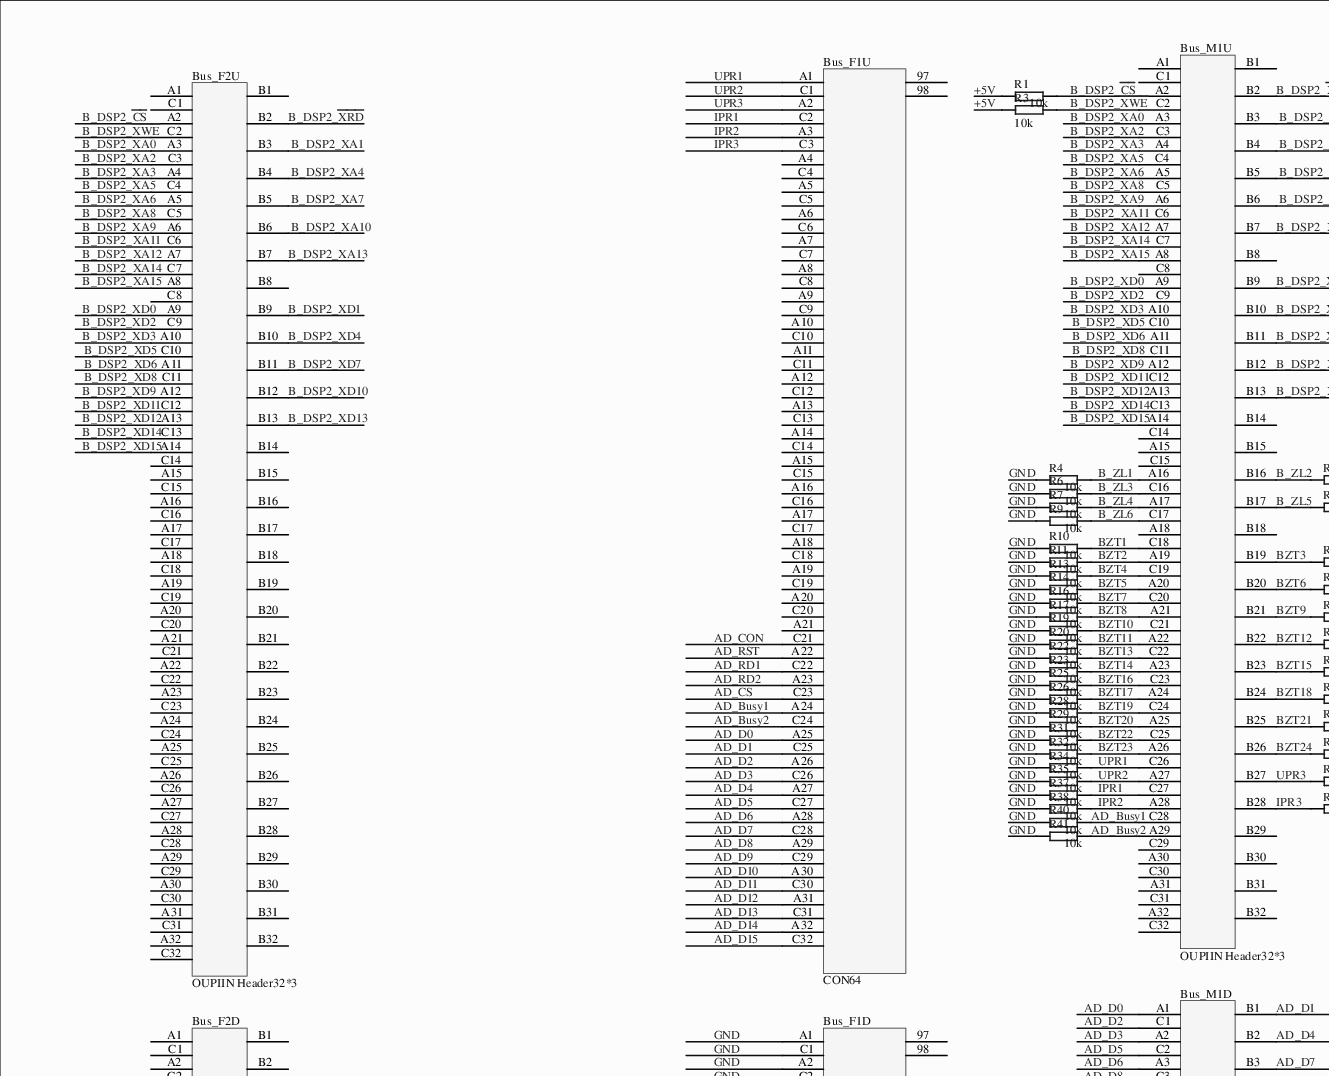
[diagram p0: MISC67337.SchDoc, top left]
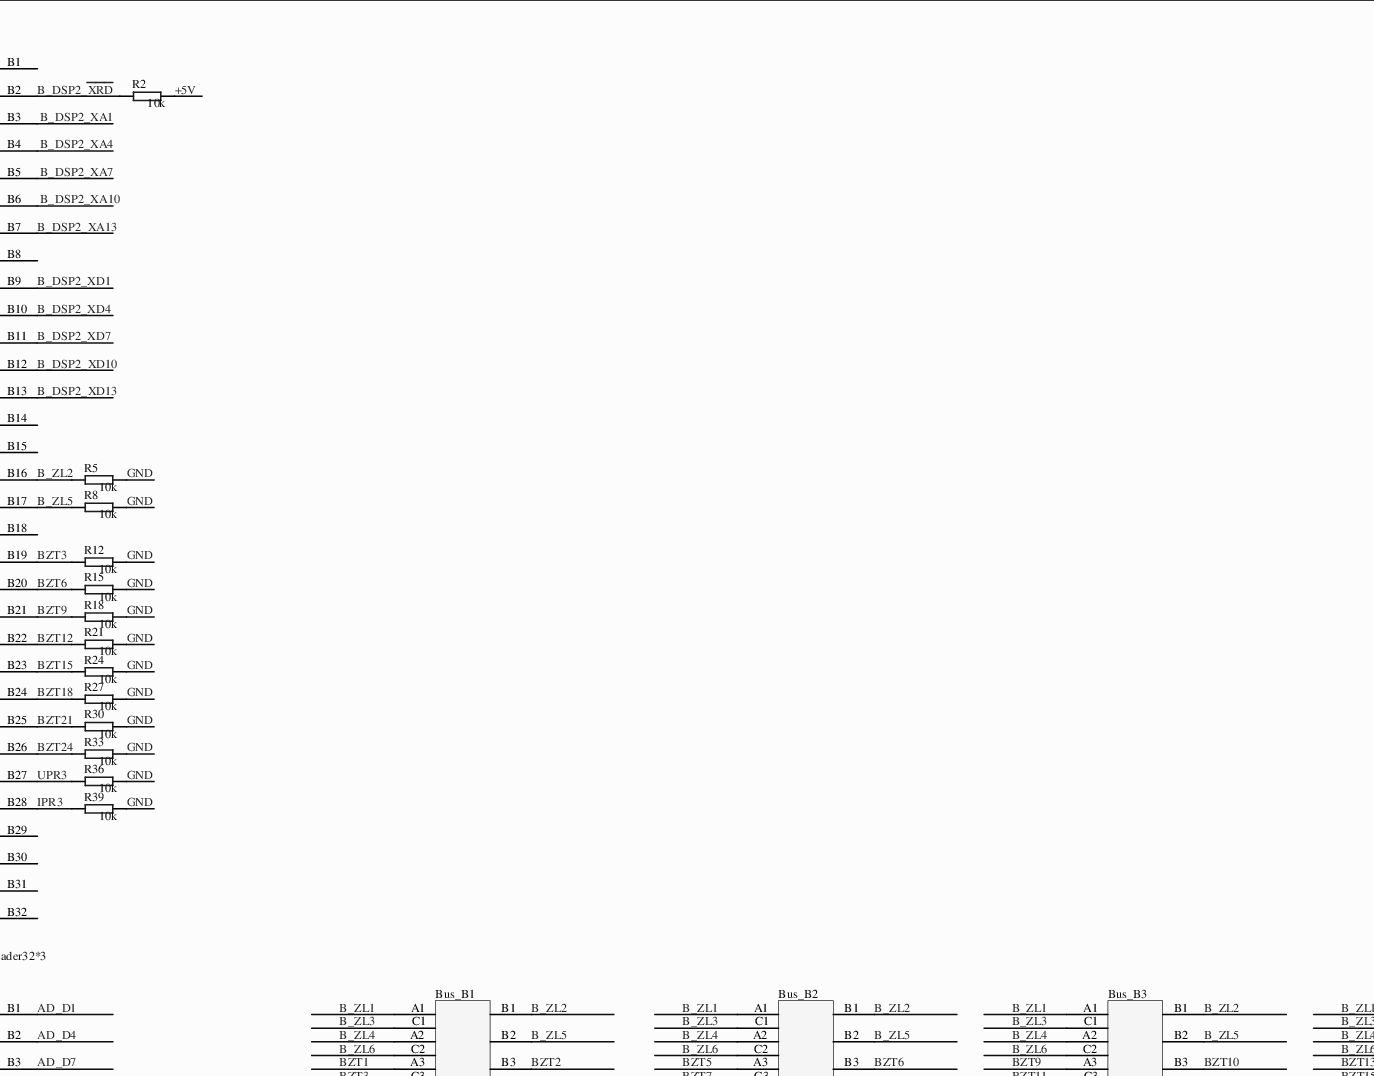
[diagram p1: MISC67337.SchDoc, top middle]
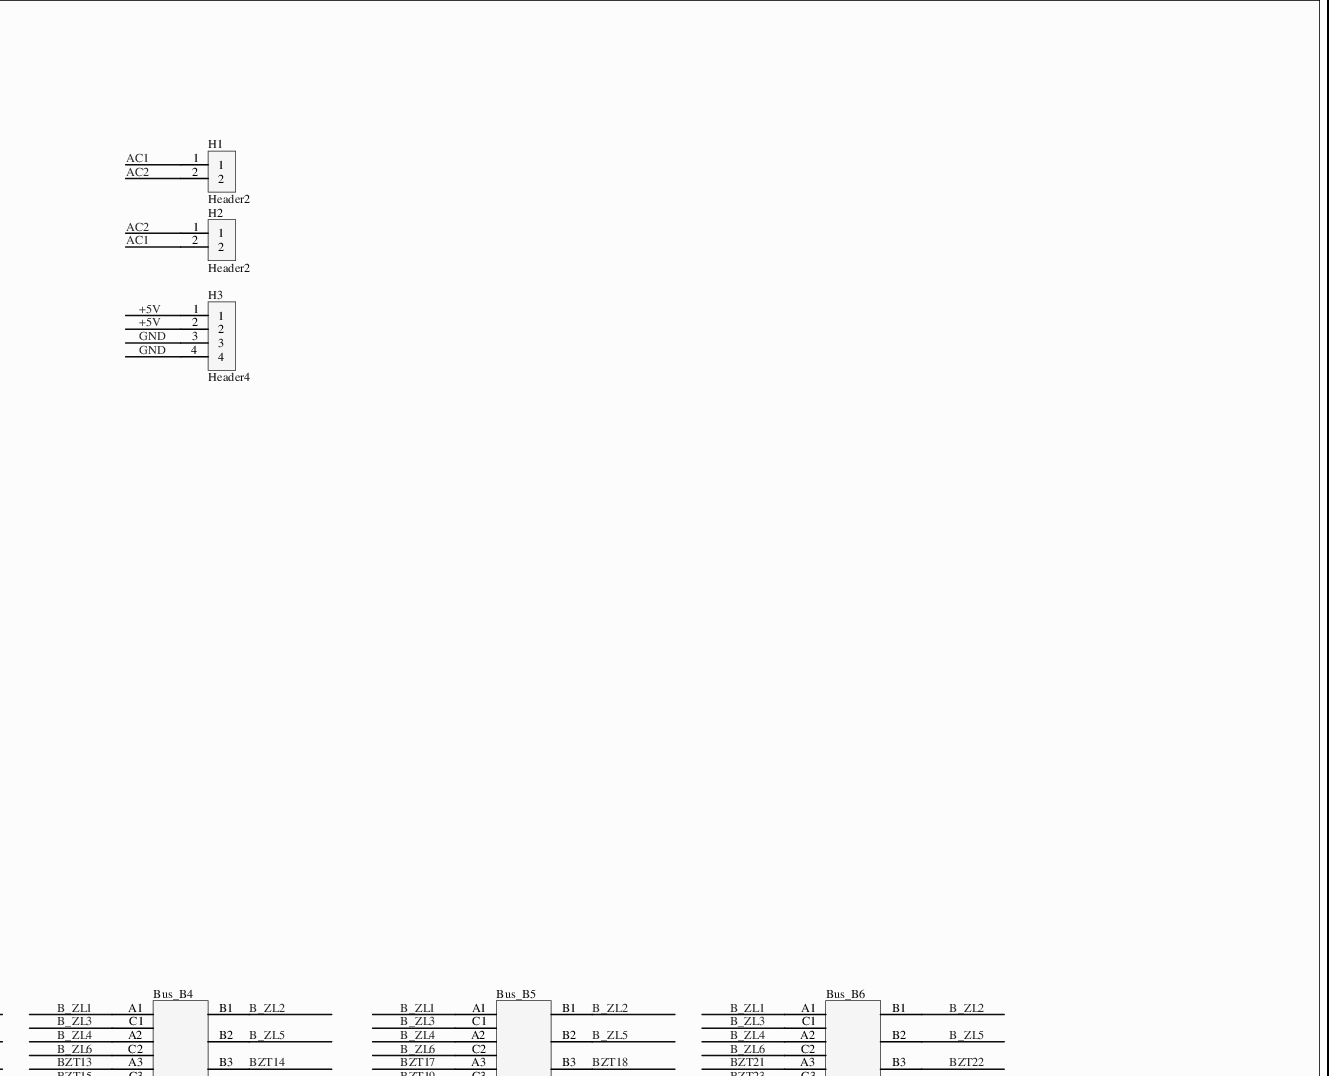
[diagram p2: MISC67337.SchDoc, top right]
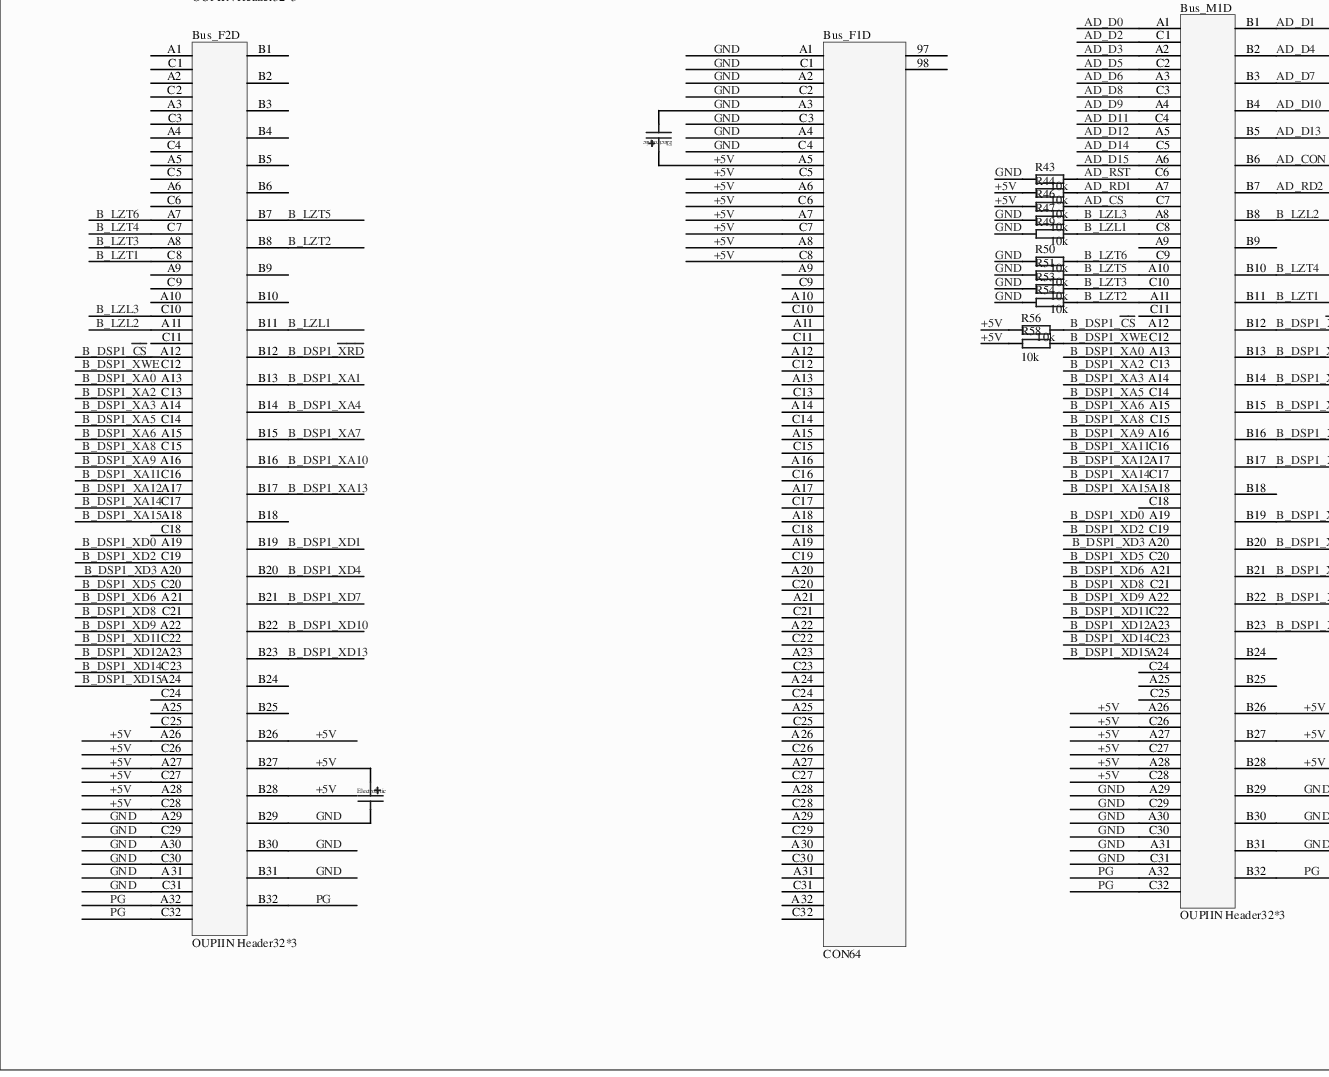
[diagram p3: MISC67337.SchDoc, bottom left]
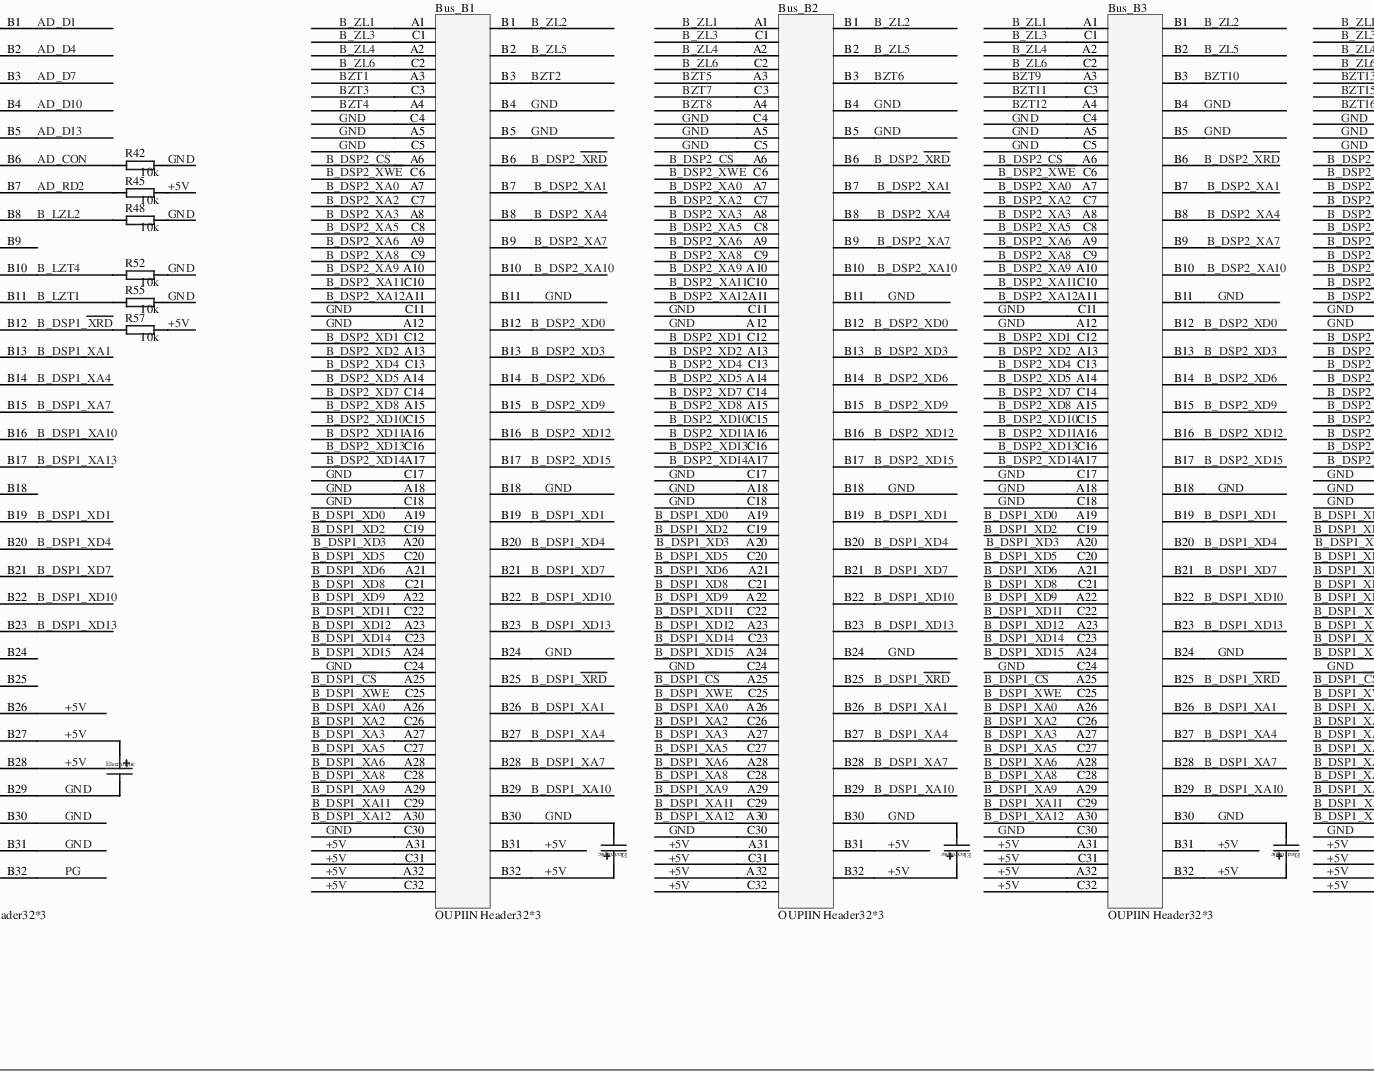
[diagram p4: MISC67337.SchDoc, bottom middle]
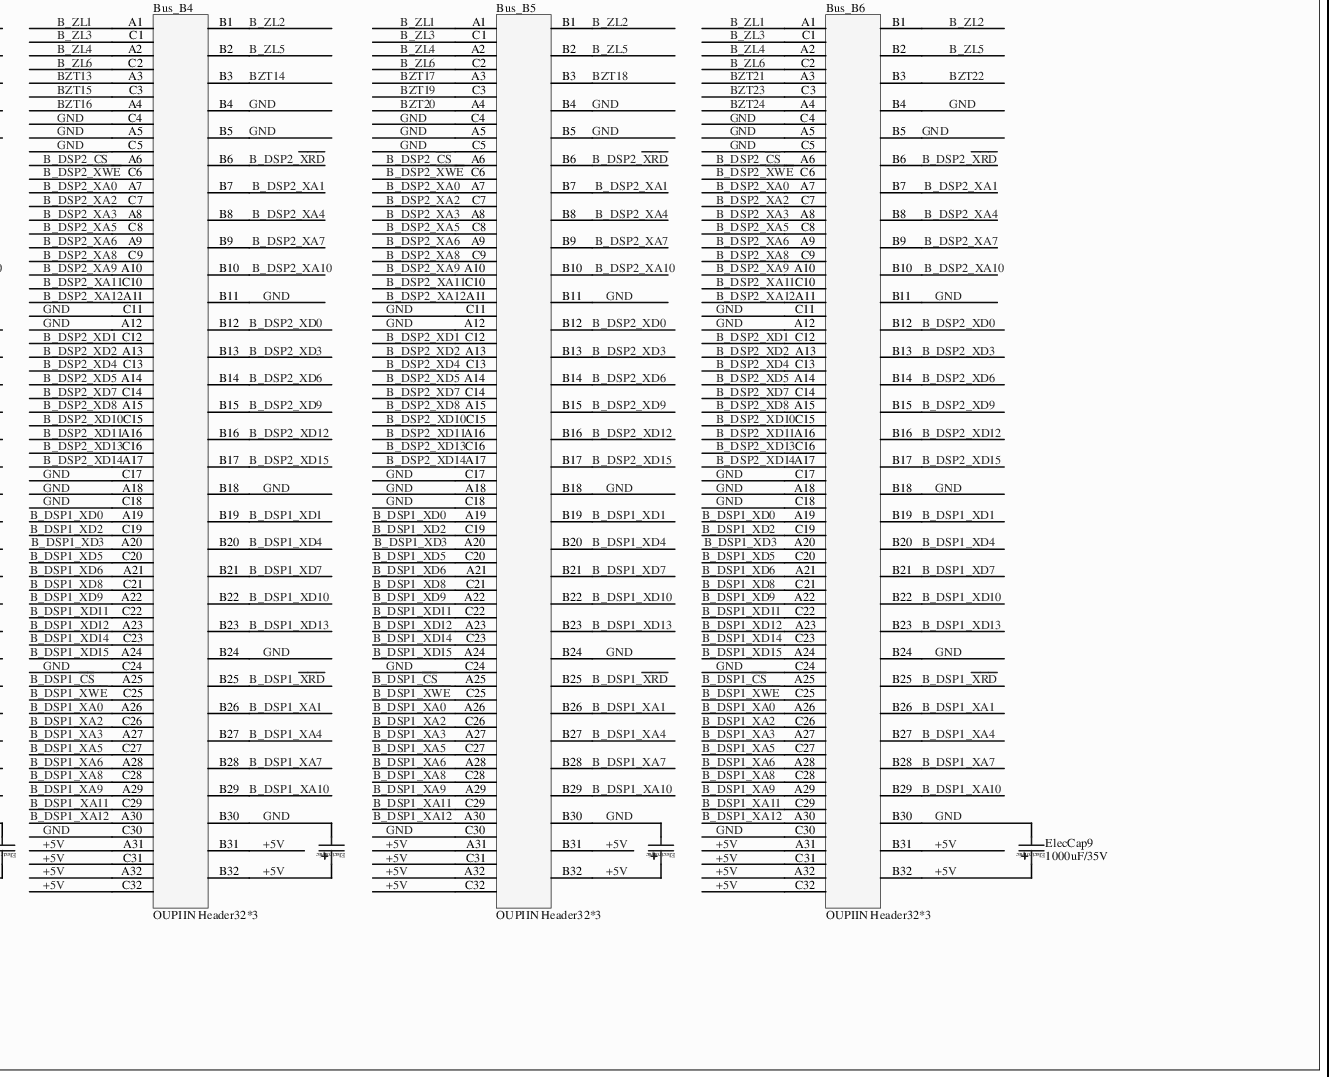
[diagram p5: MISC67337.SchDoc, bottom right]
# Altium project MISC67337.PrjPcb
1 sheet, 82 parts. Net scope: global (net labels, ports and power ports of the same name join across sheets).
Board file: MISC67337.PcbDoc

## Sheet MISC67337.SchDoc
size 711 x 381 mm; SheetNumber: 0; SheetTotal: 0

### Parts
Bus_B1  OUPIIN Header32*3  [OUPIINBus32*3_zhili]
Bus_B2  OUPIIN Header32*3  [OUPIINBus32*3_zhili]
Bus_B3  OUPIIN Header32*3  [OUPIINBus32*3_zhili]
Bus_B4  OUPIIN Header32*3  [OUPIINBus32*3_zhili]
Bus_B5  OUPIIN Header32*3  [OUPIINBus32*3_zhili]
Bus_B6  OUPIIN Header32*3  [OUPIINBus32*3_zhili]
Bus_F1D  CON64  [OUPIINBus32*2_zhili]
Bus_F1U  CON64  [OUPIINBus32*2_zhili]
Bus_F2D  OUPIIN Header32*3  [OUPIINBus32*3_zhili]
Bus_F2U  OUPIIN Header32*3  [OUPIINBus32*3_zhili]
Bus_M1D  OUPIIN Header32*3  [OUPIINBus32*3_zhili]
Bus_M1U  OUPIIN Header32*3  [OUPIINBus32*3_zhili]
ElecCap1  1000uF/35V  [1000UF/35V]  (value not drawn)
ElecCap2  1000uF/35V  [1000UF/35V]  (value not drawn)
ElecCap3  1000uF/35V  [1000UF/35V]  (value not drawn)
ElecCap4  1000uF/35V  [1000UF/35V]  (value not drawn)
ElecCap5  1000uF/35V  [1000UF/35V]  (value not drawn)
ElecCap6  1000uF/35V  [1000UF/35V]  (value not drawn)
ElecCap7  1000uF/35V  [1000UF/35V]  (value not drawn)
ElecCap8  1000uF/35V  [1000UF/35V]  (value not drawn)
ElecCap9  1000uF/35V  [1000UF/35V]
H1  Header2  [EDGCon_2p_5.08mm]
H2  Header2  [EDGCON_2p_5.08mm_ear]
H3  Header4  [EDGCON_4p_5.08mm]
R1  10k  [0603]
R2  10k  [0603]
R3  10k  [0603]
R4  10k  [0603]
R5  10k  [0603]
R6  10k  [0603]
R7  10k  [0603]
R8  10k  [0603]
R9  10k  [0603]
R10  10k  [0603]
R11  10k  [0603]
R12  10k  [0603]
R13  10k  [0603]
R14  10k  [0603]
R15  10k  [0603]
R16  10k  [0603]
R17  10k  [0603]
R18  10k  [0603]
R19  10k  [0603]
R20  10k  [0603]
R21  10k  [0603]
R22  10k  [0603]
R23  10k  [0603]
R24  10k  [0603]
R25  10k  [0603]
R26  10k  [0603]
R27  10k  [0603]
R28  10k  [0603]
R29  10k  [0603]
R30  10k  [0603]
R31  10k  [0603]
R32  10k  [0603]
R33  10k  [0603]
R34  10k  [0603]
R35  10k  [0603]
R36  10k  [0603]
R37  10k  [0603]
R38  10k  [0603]
R39  10k  [0603]
R40  10k  [0603]
R41  10k  [0603]
R42  10k  [0603]
R43  10k  [0603]
R44  10k  [0603]
R45  10k  [0603]
R46  10k  [0603]
R47  10k  [0603]
R48  10k  [0603]
R49  10k  [0603]
R50  10k  [0603]
R51  10k  [0603]
R52  10k  [0603]
R53  10k  [0603]
R54  10k  [0603]
R55  10k  [0603]
R56  10k  [0603]
R57  10k  [0603]
R58  10k  [0603]

### Nets
+5V: Bus_B1.A31 Bus_B1.A32 Bus_B1.B31 Bus_B1.B32 Bus_B1.C31 Bus_B1.C32 Bus_B2.A31 Bus_B2.A32 Bus_B2.B31 Bus_B2.B32 Bus_B2.C31 Bus_B2.C32 Bus_B3.A31 Bus_B3.A32 Bus_B3.B31 Bus_B3.B32 Bus_B3.C31 Bus_B3.C32 Bus_B4.A31 Bus_B4.A32 Bus_B4.B31 Bus_B4.B32 Bus_B4.C31 Bus_B4.C32 Bus_B5.A31 Bus_B5.A32 Bus_B5.B31 Bus_B5.B32 Bus_B5.C31 Bus_B5.C32 Bus_B6.A31 Bus_B6.A32 Bus_B6.B31 Bus_B6.B32 Bus_B6.C31 Bus_B6.C32 Bus_F1D.A5 Bus_F1D.A6 Bus_F1D.A7 Bus_F1D.A8 Bus_F1D.C5 Bus_F1D.C6 Bus_F1D.C7 Bus_F1D.C8 Bus_F2D.A26 Bus_F2D.A27 Bus_F2D.A28 Bus_F2D.B26 Bus_F2D.B27 Bus_F2D.B28 Bus_F2D.C26 Bus_F2D.C27 Bus_F2D.C28 Bus_M1D.A26 Bus_M1D.A27 Bus_M1D.A28 Bus_M1D.B26 Bus_M1D.B27 Bus_M1D.B28 Bus_M1D.C26 Bus_M1D.C27 Bus_M1D.C28 ElecCap1.1 ElecCap2.1 ElecCap3.1 ElecCap4.1 ElecCap5.1 ElecCap6.1 ElecCap7.1 ElecCap8.1 ElecCap9.1 H3.1 H3.2 R1.1 R2.2 R3.1 R44.1 R45.2 R46.1 R56.1 R57.2 R58.1
AC1: H1.1 H2.2
AC2: H1.2 H2.1
AD_Busy1: Bus_F1U.A24 Bus_M1U.C28 R40.2
AD_Busy2: Bus_F1U.C24 Bus_M1U.A29 R41.2
AD_CON: Bus_F1U.C21 Bus_M1D.B6 R42.1
AD_CS: Bus_F1U.C23 Bus_M1D.C7 R46.2
AD_D0: Bus_F1U.A25 Bus_M1D.A1
AD_D1: Bus_F1U.C25 Bus_M1D.B1
AD_D2: Bus_F1U.A26 Bus_M1D.C1
AD_D3: Bus_F1U.C26 Bus_M1D.A2
AD_D4: Bus_F1U.A27 Bus_M1D.B2
AD_D5: Bus_F1U.C27 Bus_M1D.C2
AD_D6: Bus_F1U.A28 Bus_M1D.A3
AD_D7: Bus_F1U.C28 Bus_M1D.B3
AD_D8: Bus_F1U.A29 Bus_M1D.C3
AD_D9: Bus_F1U.C29 Bus_M1D.A4
AD_D10: Bus_F1U.A30 Bus_M1D.B4
AD_D11: Bus_F1U.C30 Bus_M1D.C4
AD_D12: Bus_F1U.A31 Bus_M1D.A5
AD_D13: Bus_F1U.C31 Bus_M1D.B5
AD_D14: Bus_F1U.A32 Bus_M1D.C5
AD_D15: Bus_F1U.C32 Bus_M1D.A6
AD_RD1: Bus_F1U.C22 Bus_M1D.A7 R44.2
AD_RD2: Bus_F1U.A23 Bus_M1D.B7 R45.1
AD_RST: Bus_F1U.A22 Bus_M1D.C6 R43.2
B_DSP1_~{CS}: Bus_B1.A25 Bus_B2.A25 Bus_B3.A25 Bus_B4.A25 Bus_B5.A25 Bus_B6.A25 Bus_F2D.A12 Bus_M1D.A12 R56.2
B_DSP1_~{XRD}: Bus_B1.B25 Bus_B2.B25 Bus_B3.B25 Bus_B4.B25 Bus_B5.B25 Bus_B6.B25 Bus_F2D.B12 Bus_M1D.B12 R57.1
B_DSP1_~{XWE}: Bus_B1.C25 Bus_B2.C25 Bus_B3.C25 Bus_B4.C25 Bus_B5.C25 Bus_B6.C25 Bus_F2D.C12 Bus_M1D.C12 R58.2
B_DSP1_XA0: Bus_B1.A26 Bus_B2.A26 Bus_B3.A26 Bus_B4.A26 Bus_B5.A26 Bus_B6.A26 Bus_F2D.A13 Bus_M1D.A13
B_DSP1_XA1: Bus_B1.B26 Bus_B2.B26 Bus_B3.B26 Bus_B4.B26 Bus_B5.B26 Bus_B6.B26 Bus_F2D.B13 Bus_M1D.B13
B_DSP1_XA2: Bus_B1.C26 Bus_B2.C26 Bus_B3.C26 Bus_B4.C26 Bus_B5.C26 Bus_B6.C26 Bus_F2D.C13 Bus_M1D.C13
B_DSP1_XA3: Bus_B1.A27 Bus_B2.A27 Bus_B3.A27 Bus_B4.A27 Bus_B5.A27 Bus_B6.A27 Bus_F2D.A14 Bus_M1D.A14
B_DSP1_XA4: Bus_B1.B27 Bus_B2.B27 Bus_B3.B27 Bus_B4.B27 Bus_B5.B27 Bus_B6.B27 Bus_F2D.B14 Bus_M1D.B14
B_DSP1_XA5: Bus_B1.C27 Bus_B2.C27 Bus_B3.C27 Bus_B4.C27 Bus_B5.C27 Bus_B6.C27 Bus_F2D.C14 Bus_M1D.C14
B_DSP1_XA6: Bus_B1.A28 Bus_B2.A28 Bus_B3.A28 Bus_B4.A28 Bus_B5.A28 Bus_B6.A28 Bus_F2D.A15 Bus_M1D.A15
B_DSP1_XA7: Bus_B1.B28 Bus_B2.B28 Bus_B3.B28 Bus_B4.B28 Bus_B5.B28 Bus_B6.B28 Bus_F2D.B15 Bus_M1D.B15
B_DSP1_XA8: Bus_B1.C28 Bus_B2.C28 Bus_B3.C28 Bus_B4.C28 Bus_B5.C28 Bus_B6.C28 Bus_F2D.C15 Bus_M1D.C15
B_DSP1_XA9: Bus_B1.A29 Bus_B2.A29 Bus_B3.A29 Bus_B4.A29 Bus_B5.A29 Bus_B6.A29 Bus_F2D.A16 Bus_M1D.A16
B_DSP1_XA10: Bus_B1.B29 Bus_B2.B29 Bus_B3.B29 Bus_B4.B29 Bus_B5.B29 Bus_B6.B29 Bus_F2D.B16 Bus_M1D.B16
B_DSP1_XA11: Bus_B1.C29 Bus_B2.C29 Bus_B3.C29 Bus_B4.C29 Bus_B5.C29 Bus_B6.C29 Bus_F2D.C16 Bus_M1D.C16
B_DSP1_XA12: Bus_B1.A30 Bus_B2.A30 Bus_B3.A30 Bus_B4.A30 Bus_B5.A30 Bus_B6.A30 Bus_F2D.A17 Bus_M1D.A17
B_DSP1_XA13: Bus_F2D.B17 Bus_M1D.B17
B_DSP1_XA14: Bus_F2D.C17 Bus_M1D.C17
B_DSP1_XA15: Bus_F2D.A18 Bus_M1D.A18
B_DSP1_XD0: Bus_B1.A19 Bus_B2.A19 Bus_B3.A19 Bus_B4.A19 Bus_B5.A19 Bus_B6.A19 Bus_F2D.A19 Bus_M1D.A19
B_DSP1_XD1: Bus_B1.B19 Bus_B2.B19 Bus_B3.B19 Bus_B4.B19 Bus_B5.B19 Bus_B6.B19 Bus_F2D.B19 Bus_M1D.B19
B_DSP1_XD2: Bus_B1.C19 Bus_B2.C19 Bus_B3.C19 Bus_B4.C19 Bus_B5.C19 Bus_B6.C19 Bus_F2D.C19 Bus_M1D.C19
B_DSP1_XD3: Bus_B1.A20 Bus_B2.A20 Bus_B3.A20 Bus_B4.A20 Bus_B5.A20 Bus_B6.A20 Bus_F2D.A20 Bus_M1D.A20
B_DSP1_XD4: Bus_B1.B20 Bus_B2.B20 Bus_B3.B20 Bus_B4.B20 Bus_B5.B20 Bus_B6.B20 Bus_F2D.B20 Bus_M1D.B20
B_DSP1_XD5: Bus_B1.C20 Bus_B2.C20 Bus_B3.C20 Bus_B4.C20 Bus_B5.C20 Bus_B6.C20 Bus_F2D.C20 Bus_M1D.C20
B_DSP1_XD6: Bus_B1.A21 Bus_B2.A21 Bus_B3.A21 Bus_B4.A21 Bus_B5.A21 Bus_B6.A21 Bus_F2D.A21 Bus_M1D.A21
B_DSP1_XD7: Bus_B1.B21 Bus_B2.B21 Bus_B3.B21 Bus_B4.B21 Bus_B5.B21 Bus_B6.B21 Bus_F2D.B21 Bus_M1D.B21
B_DSP1_XD8: Bus_B1.C21 Bus_B2.C21 Bus_B3.C21 Bus_B4.C21 Bus_B5.C21 Bus_B6.C21 Bus_F2D.C21 Bus_M1D.C21
B_DSP1_XD9: Bus_B1.A22 Bus_B2.A22 Bus_B3.A22 Bus_B4.A22 Bus_B5.A22 Bus_B6.A22 Bus_F2D.A22 Bus_M1D.A22
B_DSP1_XD10: Bus_B1.B22 Bus_B2.B22 Bus_B3.B22 Bus_B4.B22 Bus_B5.B22 Bus_B6.B22 Bus_F2D.B22 Bus_M1D.B22
B_DSP1_XD11: Bus_B1.C22 Bus_B2.C22 Bus_B3.C22 Bus_B4.C22 Bus_B5.C22 Bus_B6.C22 Bus_F2D.C22 Bus_M1D.C22
B_DSP1_XD12: Bus_B1.A23 Bus_B2.A23 Bus_B3.A23 Bus_B4.A23 Bus_B5.A23 Bus_B6.A23 Bus_F2D.A23 Bus_M1D.A23
B_DSP1_XD13: Bus_B1.B23 Bus_B2.B23 Bus_B3.B23 Bus_B4.B23 Bus_B5.B23 Bus_B6.B23 Bus_F2D.B23 Bus_M1D.B23
B_DSP1_XD14: Bus_B1.C23 Bus_B2.C23 Bus_B3.C23 Bus_B4.C23 Bus_B5.C23 Bus_B6.C23 Bus_F2D.C23 Bus_M1D.C23
B_DSP1_XD15: Bus_B1.A24 Bus_B2.A24 Bus_B3.A24 Bus_B4.A24 Bus_B5.A24 Bus_B6.A24 Bus_F2D.A24 Bus_M1D.A24
B_DSP2_~{CS}: Bus_B1.A6 Bus_B2.A6 Bus_B3.A6 Bus_B4.A6 Bus_B5.A6 Bus_B6.A6 Bus_F2U.A2 Bus_M1U.A2 R1.2
B_DSP2_~{XRD}: Bus_B1.B6 Bus_B2.B6 Bus_B3.B6 Bus_B4.B6 Bus_B5.B6 Bus_B6.B6 Bus_F2U.B2 Bus_M1U.B2 R2.1
B_DSP2_~{XWE}: Bus_B1.C6 Bus_B2.C6 Bus_B3.C6 Bus_B4.C6 Bus_B5.C6 Bus_B6.C6 Bus_F2U.C2 Bus_M1U.C2 R3.2
B_DSP2_XA0: Bus_B1.A7 Bus_B2.A7 Bus_B3.A7 Bus_B4.A7 Bus_B5.A7 Bus_B6.A7 Bus_F2U.A3 Bus_M1U.A3
B_DSP2_XA1: Bus_B1.B7 Bus_B2.B7 Bus_B3.B7 Bus_B4.B7 Bus_B5.B7 Bus_B6.B7 Bus_F2U.B3 Bus_M1U.B3
B_DSP2_XA2: Bus_B1.C7 Bus_B2.C7 Bus_B3.C7 Bus_B4.C7 Bus_B5.C7 Bus_B6.C7 Bus_F2U.C3 Bus_M1U.C3
B_DSP2_XA3: Bus_B1.A8 Bus_B2.A8 Bus_B3.A8 Bus_B4.A8 Bus_B5.A8 Bus_B6.A8 Bus_F2U.A4 Bus_M1U.A4
B_DSP2_XA4: Bus_B1.B8 Bus_B2.B8 Bus_B3.B8 Bus_B4.B8 Bus_B5.B8 Bus_B6.B8 Bus_F2U.B4 Bus_M1U.B4
B_DSP2_XA5: Bus_B1.C8 Bus_B2.C8 Bus_B3.C8 Bus_B4.C8 Bus_B5.C8 Bus_B6.C8 Bus_F2U.C4 Bus_M1U.C4
B_DSP2_XA6: Bus_B1.A9 Bus_B2.A9 Bus_B3.A9 Bus_B4.A9 Bus_B5.A9 Bus_B6.A9 Bus_F2U.A5 Bus_M1U.A5
B_DSP2_XA7: Bus_B1.B9 Bus_B2.B9 Bus_B3.B9 Bus_B4.B9 Bus_B5.B9 Bus_B6.B9 Bus_F2U.B5 Bus_M1U.B5
B_DSP2_XA8: Bus_B1.C9 Bus_B2.C9 Bus_B3.C9 Bus_B4.C9 Bus_B5.C9 Bus_B6.C9 Bus_F2U.C5 Bus_M1U.C5
B_DSP2_XA9: Bus_B1.A10 Bus_B2.A10 Bus_B3.A10 Bus_B4.A10 Bus_B5.A10 Bus_B6.A10 Bus_F2U.A6 Bus_M1U.A6
B_DSP2_XA10: Bus_B1.B10 Bus_B2.B10 Bus_B3.B10 Bus_B4.B10 Bus_B5.B10 Bus_B6.B10 Bus_F2U.B6 Bus_M1U.B6
B_DSP2_XA11: Bus_B1.C10 Bus_B2.C10 Bus_B3.C10 Bus_B4.C10 Bus_B5.C10 Bus_B6.C10 Bus_F2U.C6 Bus_M1U.C6
B_DSP2_XA12: Bus_B1.A11 Bus_B2.A11 Bus_B3.A11 Bus_B4.A11 Bus_B5.A11 Bus_B6.A11 Bus_F2U.A7 Bus_M1U.A7
B_DSP2_XA13: Bus_F2U.B7 Bus_M1U.B7
B_DSP2_XA14: Bus_F2U.C7 Bus_M1U.C7
B_DSP2_XA15: Bus_F2U.A8 Bus_M1U.A8
B_DSP2_XD0: Bus_B1.B12 Bus_B2.B12 Bus_B3.B12 Bus_B4.B12 Bus_B5.B12 Bus_B6.B12 Bus_F2U.A9 Bus_M1U.A9
B_DSP2_XD1: Bus_B1.C12 Bus_B2.C12 Bus_B3.C12 Bus_B4.C12 Bus_B5.C12 Bus_B6.C12 Bus_F2U.B9 Bus_M1U.B9
B_DSP2_XD2: Bus_B1.A13 Bus_B2.A13 Bus_B3.A13 Bus_B4.A13 Bus_B5.A13 Bus_B6.A13 Bus_F2U.C9 Bus_M1U.C9
B_DSP2_XD3: Bus_B1.B13 Bus_B2.B13 Bus_B3.B13 Bus_B4.B13 Bus_B5.B13 Bus_B6.B13 Bus_F2U.A10 Bus_M1U.A10
B_DSP2_XD4: Bus_B1.C13 Bus_B2.C13 Bus_B3.C13 Bus_B4.C13 Bus_B5.C13 Bus_B6.C13 Bus_F2U.B10 Bus_M1U.B10
B_DSP2_XD5: Bus_B1.A14 Bus_B2.A14 Bus_B3.A14 Bus_B4.A14 Bus_B5.A14 Bus_B6.A14 Bus_F2U.C10 Bus_M1U.C10
B_DSP2_XD6: Bus_B1.B14 Bus_B2.B14 Bus_B3.B14 Bus_B4.B14 Bus_B5.B14 Bus_B6.B14 Bus_F2U.A11 Bus_M1U.A11
B_DSP2_XD7: Bus_B1.C14 Bus_B2.C14 Bus_B3.C14 Bus_B4.C14 Bus_B5.C14 Bus_B6.C14 Bus_F2U.B11 Bus_M1U.B11
B_DSP2_XD8: Bus_B1.A15 Bus_B2.A15 Bus_B3.A15 Bus_B4.A15 Bus_B5.A15 Bus_B6.A15 Bus_F2U.C11 Bus_M1U.C11
B_DSP2_XD9: Bus_B1.B15 Bus_B2.B15 Bus_B3.B15 Bus_B4.B15 Bus_B5.B15 Bus_B6.B15 Bus_F2U.A12 Bus_M1U.A12
B_DSP2_XD10: Bus_B1.C15 Bus_B2.C15 Bus_B3.C15 Bus_B4.C15 Bus_B5.C15 Bus_B6.C15 Bus_F2U.B12 Bus_M1U.B12
B_DSP2_XD11: Bus_B1.A16 Bus_B2.A16 Bus_B3.A16 Bus_B4.A16 Bus_B5.A16 Bus_B6.A16 Bus_F2U.C12 Bus_M1U.C12
B_DSP2_XD12: Bus_B1.B16 Bus_B2.B16 Bus_B3.B16 Bus_B4.B16 Bus_B5.B16 Bus_B6.B16 Bus_F2U.A13 Bus_M1U.A13
B_DSP2_XD13: Bus_B1.C16 Bus_B2.C16 Bus_B3.C16 Bus_B4.C16 Bus_B5.C16 Bus_B6.C16 Bus_F2U.B13 Bus_M1U.B13
B_DSP2_XD14: Bus_B1.A17 Bus_B2.A17 Bus_B3.A17 Bus_B4.A17 Bus_B5.A17 Bus_B6.A17 Bus_F2U.C13 Bus_M1U.C13
B_DSP2_XD15: Bus_B1.B17 Bus_B2.B17 Bus_B3.B17 Bus_B4.B17 Bus_B5.B17 Bus_B6.B17 Bus_F2U.A14 Bus_M1U.A14
B_LZL1: Bus_F2D.B11 Bus_M1D.C8 R49.2
B_LZL2: Bus_F2D.A11 Bus_M1D.B8 R48.1
B_LZL3: Bus_F2D.C10 Bus_M1D.A8 R47.2
B_LZT1: Bus_F2D.C8 Bus_M1D.B11 R55.1
B_LZT2: Bus_F2D.B8 Bus_M1D.A11 R54.2
B_LZT3: Bus_F2D.A8 Bus_M1D.C10 R53.2
B_LZT4: Bus_F2D.C7 Bus_M1D.B10 R52.1
B_LZT5: Bus_F2D.B7 Bus_M1D.A10 R51.2
B_LZT6: Bus_F2D.A7 Bus_M1D.C9 R50.2
B_ZL1: Bus_B1.A1 Bus_B2.A1 Bus_B3.A1 Bus_B4.A1 Bus_B5.A1 Bus_B6.A1 Bus_M1U.A16 R4.2
B_ZL2: Bus_B1.B1 Bus_B2.B1 Bus_B3.B1 Bus_B4.B1 Bus_B5.B1 Bus_B6.B1 Bus_M1U.B16 R5.1
B_ZL3: Bus_B1.C1 Bus_B2.C1 Bus_B3.C1 Bus_B4.C1 Bus_B5.C1 Bus_B6.C1 Bus_M1U.C16 R6.2
B_ZL4: Bus_B1.A2 Bus_B2.A2 Bus_B3.A2 Bus_B4.A2 Bus_B5.A2 Bus_B6.A2 Bus_M1U.A17 R7.2
B_ZL5: Bus_B1.B2 Bus_B2.B2 Bus_B3.B2 Bus_B4.B2 Bus_B5.B2 Bus_B6.B2 Bus_M1U.B17 R8.1
B_ZL6: Bus_B1.C2 Bus_B2.C2 Bus_B3.C2 Bus_B4.C2 Bus_B5.C2 Bus_B6.C2 Bus_M1U.C17 R9.2
BZT1: Bus_B1.A3 Bus_M1U.C18 R10.2
BZT2: Bus_B1.B3 Bus_M1U.A19 R11.2
BZT3: Bus_B1.C3 Bus_M1U.B19 R12.1
BZT4: Bus_B1.A4 Bus_M1U.C19 R13.2
BZT5: Bus_B2.A3 Bus_M1U.A20 R14.2
BZT6: Bus_B2.B3 Bus_M1U.B20 R15.1
BZT7: Bus_B2.C3 Bus_M1U.C20 R16.2
BZT8: Bus_B2.A4 Bus_M1U.A21 R17.2
BZT9: Bus_B3.A3 Bus_M1U.B21 R18.1
BZT10: Bus_B3.B3 Bus_M1U.C21 R19.2
BZT11: Bus_B3.C3 Bus_M1U.A22 R20.2
BZT12: Bus_B3.A4 Bus_M1U.B22 R21.1
BZT13: Bus_B4.A3 Bus_M1U.C22 R22.2
BZT14: Bus_B4.B3 Bus_M1U.A23 R23.2
BZT15: Bus_B4.C3 Bus_M1U.B23 R24.1
BZT16: Bus_B4.A4 Bus_M1U.C23 R25.2
BZT17: Bus_B5.A3 Bus_M1U.A24 R26.2
BZT18: Bus_B5.B3 Bus_M1U.B24 R27.1
BZT19: Bus_B5.C3 Bus_M1U.C24 R28.2
BZT20: Bus_B5.A4 Bus_M1U.A25 R29.2
BZT21: Bus_B6.A3 Bus_M1U.B25 R30.1
BZT22: Bus_B6.B3 Bus_M1U.C25 R31.2
BZT23: Bus_B6.C3 Bus_M1U.A26 R32.2
BZT24: Bus_B6.A4 Bus_M1U.B26 R33.1
GND: Bus_B1.A5 Bus_B1.A12 Bus_B1.A18 Bus_B1.B4 Bus_B1.B5 Bus_B1.B11 Bus_B1.B18 Bus_B1.B24 Bus_B1.B30 Bus_B1.C4 Bus_B1.C5 Bus_B1.C11 Bus_B1.C17 Bus_B1.C18 Bus_B1.C24 Bus_B1.C30 Bus_B2.A5 Bus_B2.A12 Bus_B2.A18 Bus_B2.B4 Bus_B2.B5 Bus_B2.B11 Bus_B2.B18 Bus_B2.B24 Bus_B2.B30 Bus_B2.C4 Bus_B2.C5 Bus_B2.C11 Bus_B2.C17 Bus_B2.C18 Bus_B2.C24 Bus_B2.C30 Bus_B3.A5 Bus_B3.A12 Bus_B3.A18 Bus_B3.B4 Bus_B3.B5 Bus_B3.B11 Bus_B3.B18 Bus_B3.B24 Bus_B3.B30 Bus_B3.C4 Bus_B3.C5 Bus_B3.C11 Bus_B3.C17 Bus_B3.C18 Bus_B3.C24 Bus_B3.C30 Bus_B4.A5 Bus_B4.A12 Bus_B4.A18 Bus_B4.B4 Bus_B4.B5 Bus_B4.B11 Bus_B4.B18 Bus_B4.B24 Bus_B4.B30 Bus_B4.C4 Bus_B4.C5 Bus_B4.C11 Bus_B4.C17 Bus_B4.C18 Bus_B4.C24 Bus_B4.C30 Bus_B5.A5 Bus_B5.A12 Bus_B5.A18 Bus_B5.B4 Bus_B5.B5 Bus_B5.B11 Bus_B5.B18 Bus_B5.B24 Bus_B5.B30 Bus_B5.C4 Bus_B5.C5 Bus_B5.C11 Bus_B5.C17 Bus_B5.C18 Bus_B5.C24 Bus_B5.C30 Bus_B6.A5 Bus_B6.A12 Bus_B6.A18 Bus_B6.B4 Bus_B6.B5 Bus_B6.B11 Bus_B6.B18 Bus_B6.B24 Bus_B6.B30 Bus_B6.C4 Bus_B6.C5 Bus_B6.C11 Bus_B6.C17 Bus_B6.C18 Bus_B6.C24 Bus_B6.C30 Bus_F1D.A1 Bus_F1D.A2 Bus_F1D.A3 Bus_F1D.A4 Bus_F1D.C1 Bus_F1D.C2 Bus_F1D.C3 Bus_F1D.C4 Bus_F2D.A29 Bus_F2D.A30 Bus_F2D.A31 Bus_F2D.B29 Bus_F2D.B30 Bus_F2D.B31 Bus_F2D.C29 Bus_F2D.C30 Bus_F2D.C31 Bus_M1D.A29 Bus_M1D.A30 Bus_M1D.A31 Bus_M1D.B29 Bus_M1D.B30 Bus_M1D.B31 Bus_M1D.C29 Bus_M1D.C30 Bus_M1D.C31 ElecCap1.2 ElecCap2.2 ElecCap3.2 ElecCap4.2 ElecCap5.2 ElecCap6.2 ElecCap7.2 ElecCap8.2 ElecCap9.2 H3.3 H3.4 R4.1 R5.2 R6.1 R7.1 R8.2 R9.1 R10.1 R11.1 R12.2 R13.1 R14.1 R15.2 R16.1 R17.1 R18.2 R19.1 R20.1 R21.2 R22.1 R23.1 R24.2 R25.1 R26.1 R27.2 R28.1 R29.1 R30.2 R31.1 R32.1 R33.2 R34.1 R35.1 R36.2 R37.1 R38.1 R39.2 R40.1 R41.1 R42.2 R43.1 R47.1 R48.2 R49.1 R50.1 R51.1 R52.2 R53.1 R54.1 R55.2
IPR1: Bus_F1U.C2 Bus_M1U.C27 R37.2
IPR2: Bus_F1U.A3 Bus_M1U.A28 R38.2
IPR3: Bus_F1U.C3 Bus_M1U.B28 R39.1
PG: Bus_F2D.A32 Bus_F2D.B32 Bus_F2D.C32 Bus_M1D.A32 Bus_M1D.B32 Bus_M1D.C32
UPR1: Bus_F1U.A1 Bus_M1U.C26 R34.2
UPR2: Bus_F1U.C1 Bus_M1U.A27 R35.2
UPR3: Bus_F1U.A2 Bus_M1U.B27 R36.1

Not connected (* = marked no-connect by the designer): Bus_F1D 97 98 A9 A10 A11 A12 A13 A14 A15 A16 A17 A18 A19 A20 A21 A22 A23 A24 A25 A26 A27 A28 A29 A30 A31 A32 C9 C10 C11 C12 C13 C14 C15 C16 C17 C18 C19 C20 C21 C22 C23 C24 C25 C26 C27 C28 C29 C30 C31 C32; Bus_F1U 97 98 A4 A5 A6 A7 A8 A9 A10 A11 A12 A13 A14 A15 A16 A17 A18 A19 A20 A21 C4 C5 C6 C7 C8 C9 C10 C11 C12 C13 C14 C15 C16 C17 C18 C19 C20; Bus_F2D A1 A2 A3 A4 A5 A6 A9 A10 A25 B1 B2 B3 B4 B5 B6 B9 B10 B18 B24 B25 C1 C2 C3 C4 C5 C6 C9 C11 C18 C24 C25; Bus_F2U A1 A15 A16 A17 A18 A19 A20 A21 A22 A23 A24 A25 A26 A27 A28 A29 A30 A31 A32 B1 B8 B14 B15 B16 B17 B18 B19 B20 B21 B22 B23 B24 B25 B26 B27 B28 B29 B30 B31 B32 C1 C8 C14 C15 C16 C17 C18 C19 C20 C21 C22 C23 C24 C25 C26 C27 C28 C29 C30 C31 C32; Bus_M1D A9 A25 B9 B18 B24 B25 C11 C18 C24 C25; Bus_M1U A1 A15 A18 A30 A31 A32 B1 B8 B14 B15 B18 B29 B30 B31 B32 C1 C8 C14 C15 C29 C30 C31 C32

### Library data of the parts
Bus_F1D Bus_F1U = CON64: Euro-style pin header 64-pos
ElecCap1-ElecCap9 = ELECTROCap: Electrolytic Capacitor(Pin1 Positive)
R1-R58 = RES2